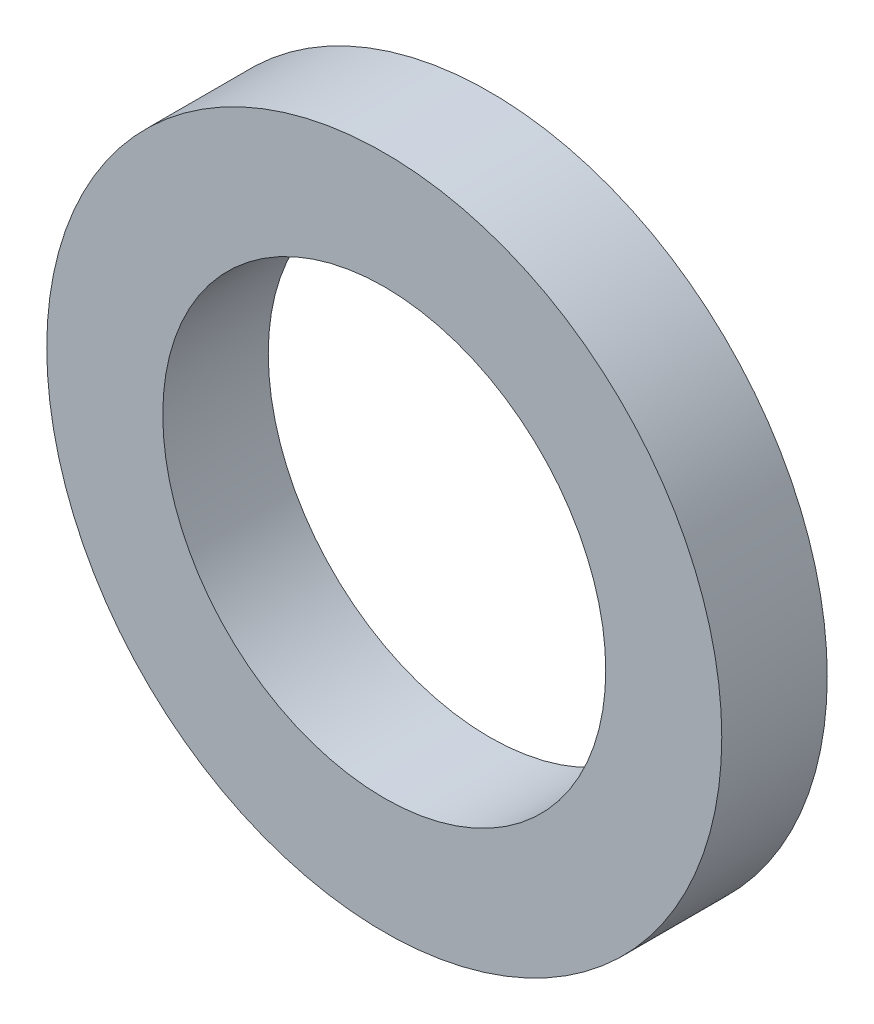
from build123d import *

# Parameters (mm, degrees)
SKETCH1_R           = 1.6
SKETCH1_R_2         = 1.05
BOSS_EXTRUDE1_DEPTH = 0.25


with BuildPart() as part:
    # Sketch1 → Boss-Extrude1 (new, symmetric)
    with BuildSketch(Plane.XY):
        Circle(SKETCH1_R)
        Circle(SKETCH1_R_2, mode=Mode.SUBTRACT)
    extrude(amount=BOSS_EXTRUDE1_DEPTH, both=True)


solid = part.part
